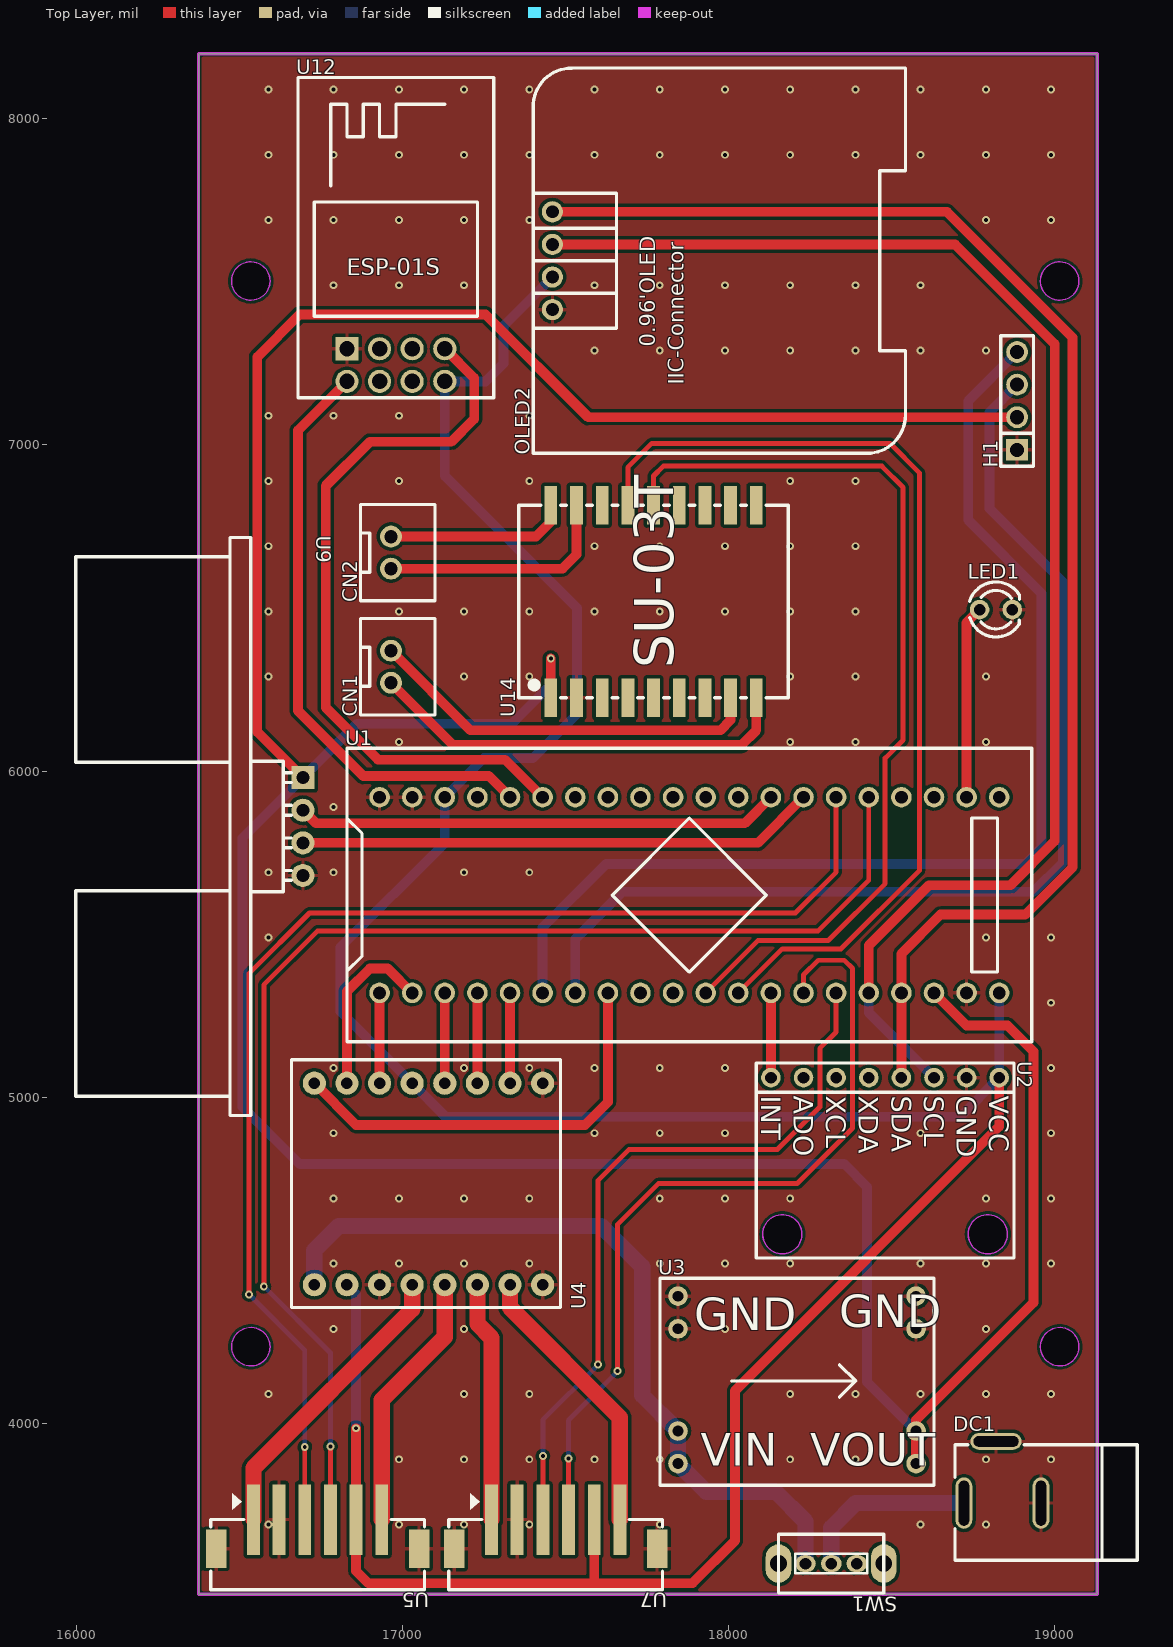
[diagram p0: Top Layer view]
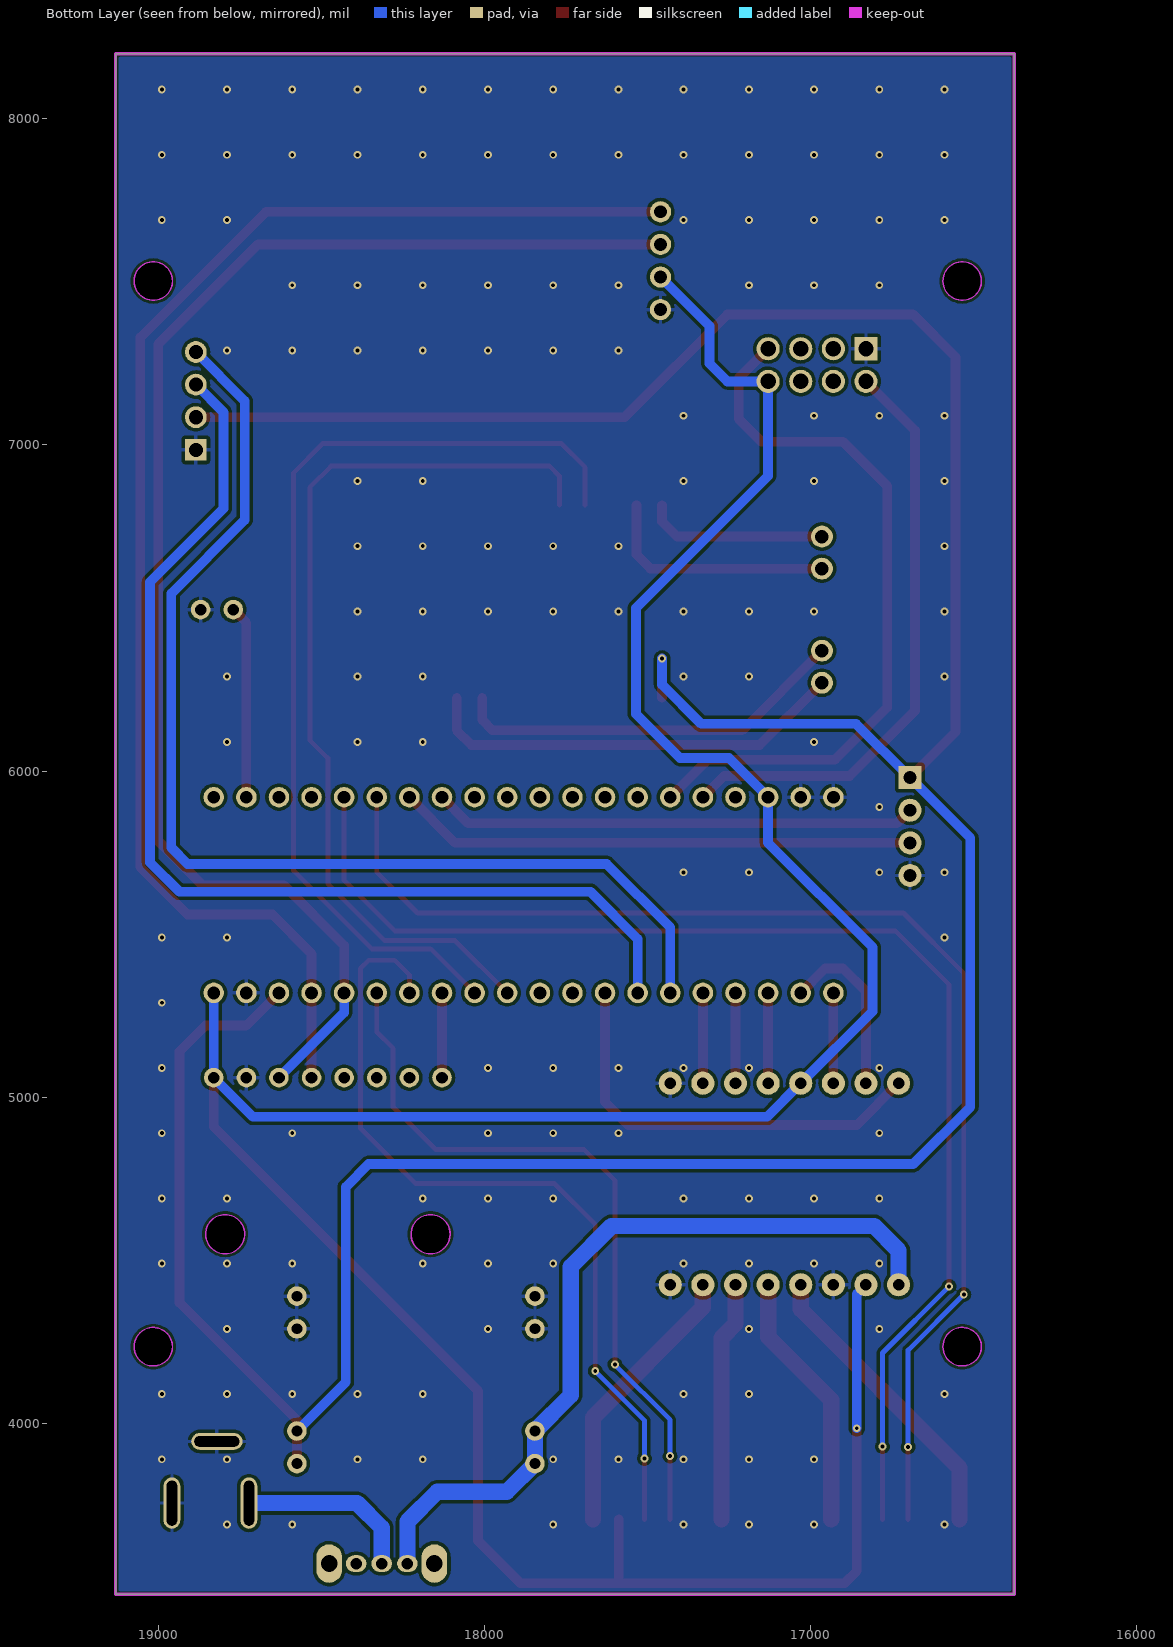
[diagram p1: Bottom Layer view, seen from below]
# Altium PCB MISC61229.pcbdoc
Units mil, origin at the board's own origin, x right, y up, seen from the top; angles counter-clockwise.
Board outline 2755.91 x 4724.41 mil, 2 copper layers (Top Layer, Bottom Layer), stack 62.206 mil thick; 16 components, 47 nets, 140 pads, 162 vias.

## Layer stack, top to bottom
Top Solder Mask Layer: solder mask 0.394, Dk 3.3
Top Layer: signal copper 1.379
Dielectric1: surface 59.449, FR4, Dk 4.5
Bottom Layer: signal copper 1.378
Bottom Solder Mask Layer: solder mask 0.394, Dk 3.3

## Board outline
16375,8200 16375,3475.59 19130.91,3475.59 19130.91,8200
cut-out: 16594.06,4235 cw(c16535,4235) 16475.94,4235 cw(c16535,4235)
cut-out: 16594.06,7502.72 cw(c16535,7502.72) 16475.94,7502.72 cw(c16535,7502.72)
cut-out: 19074.37,4235 cw(c19015.31,4235) 18956.26,4235 cw(c19015.31,4235)
cut-out: 19074.37,7502.72 cw(c19015.31,7502.72) 18956.26,7502.72 cw(c19015.31,7502.72)

## Design rules (kind name [scope] priority, off if disabled: settings)
BoardOutlineClearance copperThickness2oz_1 [All] p2 off: genericclearance=7.99 ignorepadtopadclearanceinfootprint=FALSE except(0: Arc-SplitContinuation Track-SplitContinuation SMDPad-SplitContinuation THPad-SplitContinuation Via-SplitContinuation Fill-SplitContinuation Region-SplitContinuation Poly-SplitContinuation Text-SplitContinuation Hole-SplitContinuation; 5.98: Arc-CutoutEdge Track-CutoutEdge SMDPad-CutoutEdge THPad-CutoutEdge Via-CutoutEdge Text-CutoutEdge; 6.9: Hole-OutlineEdge Hole-CutoutEdge; 10: Poly-OutlineEdge Poly-CutoutEdge; 11.81: Arc-OutlineEdge Track-OutlineEdge SMDPad-OutlineEdge THPad-OutlineEdge Via-OutlineEdge Fill-OutlineEdge Region-OutlineEdge Text-OutlineEdge Fill-CutoutEdge Region-CutoutEdge)
BoardOutlineClearance Plane_innerPlane_1 [All] p4 off: genericclearance=4.02 ignorepadtopadclearanceinfootprint=FALSE except(0: Arc-SplitContinuation Track-SplitContinuation SMDPad-SplitContinuation THPad-SplitContinuation Via-SplitContinuation Fill-SplitContinuation Region-SplitContinuation Poly-SplitContinuation Text-SplitContinuation Hole-SplitContinuation; 5.98: Arc-CutoutEdge Track-CutoutEdge SMDPad-CutoutEdge THPad-CutoutEdge Via-CutoutEdge Text-CutoutEdge; 6.9: Hole-OutlineEdge Hole-CutoutEdge; 10: Poly-OutlineEdge Poly-CutoutEdge; 11.81: Arc-OutlineEdge Track-OutlineEdge SMDPad-OutlineEdge THPad-OutlineEdge Via-OutlineEdge Fill-OutlineEdge Region-OutlineEdge Text-OutlineEdge Fill-CutoutEdge Region-CutoutEdge)
BoardOutlineClearance Copper_copperRegion_1 [All] p6 off: genericclearance=4.02 ignorepadtopadclearanceinfootprint=FALSE except(0: Arc-SplitContinuation Track-SplitContinuation SMDPad-SplitContinuation THPad-SplitContinuation Via-SplitContinuation Fill-SplitContinuation Region-SplitContinuation Poly-SplitContinuation Text-SplitContinuation Hole-SplitContinuation; 5.98: Arc-CutoutEdge Track-CutoutEdge SMDPad-CutoutEdge THPad-CutoutEdge Via-CutoutEdge Text-CutoutEdge; 6.9: Hole-OutlineEdge Hole-CutoutEdge; 10: Poly-OutlineEdge Poly-CutoutEdge; 11.81: Arc-OutlineEdge Track-OutlineEdge SMDPad-OutlineEdge THPad-OutlineEdge Via-OutlineEdge Fill-OutlineEdge Region-OutlineEdge Text-OutlineEdge Fill-CutoutEdge Region-CutoutEdge)
BoardOutlineClearance Copper_copperRegion_copperThickness1oz_1 [All] p8 off: genericclearance=4.02 ignorepadtopadclearanceinfootprint=FALSE except(0: Arc-SplitContinuation Track-SplitContinuation SMDPad-SplitContinuation THPad-SplitContinuation Via-SplitContinuation Fill-SplitContinuation Region-SplitContinuation Poly-SplitContinuation Text-SplitContinuation Hole-SplitContinuation; 5.98: Arc-CutoutEdge Track-CutoutEdge SMDPad-CutoutEdge THPad-CutoutEdge Via-CutoutEdge Text-CutoutEdge; 6.9: Hole-OutlineEdge Hole-CutoutEdge; 10: Poly-OutlineEdge Poly-CutoutEdge; 11.81: Arc-OutlineEdge Track-OutlineEdge SMDPad-OutlineEdge THPad-OutlineEdge Via-OutlineEdge Fill-OutlineEdge Region-OutlineEdge Text-OutlineEdge Fill-CutoutEdge Region-CutoutEdge)
BoardOutlineClearance Copper_copperRegion_Copper_copperRegion_1 [All] p10 off: genericclearance=4.02 ignorepadtopadclearanceinfootprint=FALSE except(0: Arc-SplitContinuation Track-SplitContinuation SMDPad-SplitContinuation THPad-SplitContinuation Via-SplitContinuation Fill-SplitContinuation Region-SplitContinuation Poly-SplitContinuation Text-SplitContinuation Hole-SplitContinuation; 5.98: Arc-CutoutEdge Track-CutoutEdge SMDPad-CutoutEdge THPad-CutoutEdge Via-CutoutEdge Text-CutoutEdge; 6.9: Hole-OutlineEdge Hole-CutoutEdge; 10: Poly-OutlineEdge Poly-CutoutEdge; 11.81: Arc-OutlineEdge Track-OutlineEdge SMDPad-OutlineEdge THPad-OutlineEdge Via-OutlineEdge Fill-OutlineEdge Region-OutlineEdge Text-OutlineEdge Fill-CutoutEdge Region-CutoutEdge)
BoardOutlineClearance copperThickness1oz_1 [All] p12: genericclearance=4.02 ignorepadtopadclearanceinfootprint=FALSE except(0: Arc-SplitContinuation Track-SplitContinuation SMDPad-SplitContinuation THPad-SplitContinuation Via-SplitContinuation Fill-SplitContinuation Region-SplitContinuation Poly-SplitContinuation Text-SplitContinuation Hole-SplitContinuation; 5.98: Arc-CutoutEdge Track-CutoutEdge SMDPad-CutoutEdge THPad-CutoutEdge Via-CutoutEdge Text-CutoutEdge; 6.9: Hole-OutlineEdge Hole-CutoutEdge; 10: Poly-OutlineEdge Poly-CutoutEdge; 11.81: Arc-OutlineEdge Track-OutlineEdge SMDPad-OutlineEdge THPad-OutlineEdge Via-OutlineEdge Fill-OutlineEdge Region-OutlineEdge Text-OutlineEdge Fill-CutoutEdge Region-CutoutEdge)
Clearance copperThickness2oz [All] p1 off: gap=7.99 ignorepadtopadclearanceinfootprint=FALSE except(5.98: SMDPad-Track SMDPad-SMDPad THPad-Track SMDPad-THPad THPad-THPad Track-Via SMDPad-Via THPad-Via Via-Via Fill-SMDPad Region-SMDPad Fill-THPad Region-THPad Fill-Via Region-Via Fill-Fill Fill-Region Region-Region Arc-Track Arc-SMDPad Arc-THPad Arc-Via Fill-Arc Region-Arc Arc-Arc Text-Track SMDPad-Text Text-THPad Text-Via Fill-Text Region-Text Arc-Text Text-Text; 6.9: Hole-Track Hole-SMDPad Hole-THPad Hole-Via Fill-Hole Region-Hole Hole-Arc Hole-Text; 10: Poly-Track Poly-SMDPad Poly-THPad Poly-Via Poly-Fill Poly-Region Poly-Poly Poly-Arc Poly-Text Poly-Hole; 11.81: Fill-Track Region-Track)
Clearance Plane_innerPlane [All] p3 off: gap=4.02 ignorepadtopadclearanceinfootprint=FALSE except(5.98: SMDPad-Track SMDPad-SMDPad THPad-Track SMDPad-THPad THPad-THPad Track-Via SMDPad-Via THPad-Via Via-Via Fill-SMDPad Region-SMDPad Fill-THPad Region-THPad Fill-Via Region-Via Fill-Fill Fill-Region Region-Region Arc-Track Arc-SMDPad Arc-THPad Arc-Via Fill-Arc Region-Arc Arc-Arc Text-Track SMDPad-Text Text-THPad Text-Via Fill-Text Region-Text Arc-Text Text-Text; 6.9: Hole-Track Hole-SMDPad Hole-THPad Hole-Via Fill-Hole Region-Hole Hole-Arc Hole-Text; 10: Poly-Track Poly-SMDPad Poly-THPad Poly-Via Poly-Fill Poly-Region Poly-Poly Poly-Arc Poly-Text Poly-Hole; 11.81: Fill-Track Region-Track)
Clearance Copper_copperRegion [All] p5 off: gap=4.02 ignorepadtopadclearanceinfootprint=FALSE except(5.98: SMDPad-Track SMDPad-SMDPad THPad-Track SMDPad-THPad THPad-THPad Track-Via SMDPad-Via THPad-Via Via-Via Fill-SMDPad Region-SMDPad Fill-THPad Region-THPad Fill-Via Region-Via Fill-Fill Fill-Region Region-Region Arc-Track Arc-SMDPad Arc-THPad Arc-Via Fill-Arc Region-Arc Arc-Arc Text-Track SMDPad-Text Text-THPad Text-Via Fill-Text Region-Text Arc-Text Text-Text; 6.9: Hole-Track Hole-SMDPad Hole-THPad Hole-Via Fill-Hole Region-Hole Hole-Arc Hole-Text; 10: Poly-Track Poly-SMDPad Poly-THPad Poly-Via Poly-Fill Poly-Region Poly-Poly Poly-Arc Poly-Text Poly-Hole; 11.81: Fill-Track Region-Track)
Clearance Copper_copperRegion_copperThickness1oz [All] p7 off: gap=4.02 ignorepadtopadclearanceinfootprint=FALSE except(5.98: SMDPad-Track SMDPad-SMDPad THPad-Track SMDPad-THPad THPad-THPad Track-Via SMDPad-Via THPad-Via Via-Via Fill-SMDPad Region-SMDPad Fill-THPad Region-THPad Fill-Via Region-Via Fill-Fill Fill-Region Region-Region Arc-Track Arc-SMDPad Arc-THPad Arc-Via Fill-Arc Region-Arc Arc-Arc Text-Track SMDPad-Text Text-THPad Text-Via Fill-Text Region-Text Arc-Text Text-Text; 6.9: Hole-Track Hole-SMDPad Hole-THPad Hole-Via Fill-Hole Region-Hole Hole-Arc Hole-Text; 10: Poly-Track Poly-SMDPad Poly-THPad Poly-Via Poly-Fill Poly-Region Poly-Poly Poly-Arc Poly-Text Poly-Hole; 11.81: Fill-Track Region-Track)
Clearance Copper_copperRegion_Copper_copperRegion [All] p9 off: gap=4.02 ignorepadtopadclearanceinfootprint=FALSE except(5.98: SMDPad-Track SMDPad-SMDPad THPad-Track SMDPad-THPad THPad-THPad Track-Via SMDPad-Via THPad-Via Via-Via Fill-SMDPad Region-SMDPad Fill-THPad Region-THPad Fill-Via Region-Via Fill-Fill Fill-Region Region-Region Arc-Track Arc-SMDPad Arc-THPad Arc-Via Fill-Arc Region-Arc Arc-Arc Text-Track SMDPad-Text Text-THPad Text-Via Fill-Text Region-Text Arc-Text Text-Text; 6.9: Hole-Track Hole-SMDPad Hole-THPad Hole-Via Fill-Hole Region-Hole Hole-Arc Hole-Text; 10: Poly-Track Poly-SMDPad Poly-THPad Poly-Via Poly-Fill Poly-Region Poly-Poly Poly-Arc Poly-Text Poly-Hole; 11.81: Fill-Track Region-Track)
Clearance copperThickness1oz [All] p11: gap=4.02 ignorepadtopadclearanceinfootprint=FALSE except(5.98: SMDPad-Track SMDPad-SMDPad THPad-Track SMDPad-THPad THPad-THPad Track-Via SMDPad-Via THPad-Via Via-Via Fill-SMDPad Region-SMDPad Fill-THPad Region-THPad Fill-Via Region-Via Fill-Fill Fill-Region Region-Region Arc-Track Arc-SMDPad Arc-THPad Arc-Via Fill-Arc Region-Arc Arc-Arc Text-Track SMDPad-Text Text-THPad Text-Via Fill-Text Region-Text Arc-Text Text-Text; 6.9: Hole-Track Hole-SMDPad Hole-THPad Hole-Via Fill-Hole Region-Hole Hole-Arc Hole-Text; 10: Poly-Track Poly-SMDPad Poly-THPad Poly-Via Poly-Fill Poly-Region Poly-Poly Poly-Arc Poly-Text Poly-Hole; 11.81: Fill-Track Region-Track)
DiffPairsRouting differentialPair [All] p1: maxlimit=6 minlimit=6 mostfreqgap=6 toplayer_minwidth=5 toplayer_prefwidth=10 toplayer_maxwidth=100 toplayer_mingap=6 toplayer_prefgap=6 toplayer_maxgap=6 bottomlayer_minwidth=5 bottomlayer_prefwidth=10 bottomlayer_maxwidth=100 bottomlayer_mingap=6 bottomlayer_prefgap=6 bottomlayer_maxgap=6 maxuncoupledlength=10
HoleToHoleClearance otherClearance [All] p1: gap=11.81 allowstackedmicrovias=TRUE
Length netLength [All] p1: minlimit=0 maxlimit=0
PasteMaskExpansion pasteMaskExpansion [All] p1: expansion=0
PlaneConnect innerPlane [All] p1: planeconnectstyle=Relief reliefexpansion=20 reliefentries=4 reliefconductorwidth=10 reliefairgap=10
PolygonConnect copperRegion_copperThickness1oz [All] p1 off: connectstyle=Relief reliefconductorwidth=10 reliefentries=4 polygonreliefangle="90 Angle" airgapwidth=10 via.connectstyle=Relief via.reliefconductorwidth=10 via.reliefentries=4 via.polygonreliefangle="90 Angle" via.airgapwidth=10
PolygonConnect copperRegion_Copper_copperRegion [All] p2 off: connectstyle=Relief reliefconductorwidth=10 reliefentries=4 polygonreliefangle="90 Angle" airgapwidth=10 via.connectstyle=Relief via.reliefconductorwidth=10 via.reliefentries=4 via.polygonreliefangle="90 Angle" via.airgapwidth=10
PolygonConnect copperRegion [All] p3: connectstyle=Relief reliefconductorwidth=10 reliefentries=4 polygonreliefangle="90 Angle" airgapwidth=10 via.connectstyle=Relief via.reliefconductorwidth=10 via.reliefentries=4 via.polygonreliefangle="90 Angle" via.airgapwidth=10
RoutingVias viaSize [All] p1: holewidth=12.01 width=24.02 viastyle="Through Hole" minholewidth=11.81 minwidth=19.68 maxholewidth=248.03 maxwidth=393.7
SolderMaskExpansion solderMaskExpansion [IsVia] p1: expansion=-1000 istentingtop=TRUE
SolderMaskExpansion solderMaskExpansion [All] p2: expansion=2 istentingtop=FALSE
Width copperThickness2oz_2 [All] p1 off: maxlimit=100 minlimit=8 preferedwidth=10
Width copperThickness1oz_2 [All] p2: maxlimit=100 minlimit=5 preferedwidth=10

## Components (designator, comment, footprint, x,y, rotation, side; value= is the part's Value field where it differs from the comment)
CN1 "XH2.54*2P_through-hole" CONN-TH_2P-P2.50-XH2.54-2P 16965,6320 r90 top
CN2 "XH2.54*2P_through-hole" CONN-TH_2P-P2.50-XH2.54-2P 16965,6670 r90 top
DC1 "" DC-2.0 18845,3745 r0 top
H1 "" HDR-TH_4P-P2.54-V-M 18884.82,7135.12 r90 top
LED1 "" LED_TH-3mm 18820,6495 r0 top
OLED2 "" 0.96OLED_4P 17460,7565 r90 top
SW1 "" 拨动开关 18320,3570 r180 top
U1 "STM32F103C8T6-Card" CONN-TH_L53.3-W22.9_STM32F103C8T6-CARD 17880,5620 r0 top
U2 "MPU6050 module" MPU6050 18480,5060 r270 top
U3 "" MP1584主控 17845,4390 r0 top
U4 "" tb6612 16730,4425 r90 top
U5 "MXPH-2.0-06P-LT1-0-A" CONN-SMD_6P-P2.00_MXPH-2.0-6P-LT1-0-A 16740,3660 r180 top
U7 "MXPH-2.0-06P-LT1-0-A" CONN-SMD_6P-P2.00_MXPH-2.0-6P-LT1-0-A 17470,3660 r180 top
U9 "HC-SR04" TH_HC-SR04V 16695,5830 r270 top
U12 "ESP-01S" WIFIM-TH_ESP-01S 16980,7245 r0 top
U14 "" SU-03T 18085,6520 r90 top

## Footprints (in the part's own frame and the unit in brackets; to place one, negate y for a bottom-side part, rotate by r counter-clockwise, add the part's x,y. Pads: shape width x height; smd on the part's side, far side on the other; paste and mask are expansions set on the pad)
0.96OLED_4P [mm]
  round 1.65 hole 1 copper offset 0,0: 1(-3.81,-0.001) 2(-1.27,0.002) 3(1.27,0.002) 4(3.81,0.002)
  silkscreen extent -15,-27.5 15,1.5
CONN-SMD_6P-P2.00_MXPH-2.0-6P-LT1-0-A [mm]
  rect 1x5.5 smd paste+0 mask+0.05: 1(5,-1.14) 2(3,-1.14) 3(1,-1.14) 4(-1,-1.14) 5(-3,-1.14) 6(-5,-1.14)
  rect 1.6x3 smd paste+0 mask+0.05: 7(-7.9,1.14) 8(7.9,1.14)
  silkscreen extent -8.32,-3.17 8.32,4.32
CONN-TH_2P-P2.50-XH2.54-2P [mm]
  round 1.7 hole 1.05 paste+0 mask+0.05: 1(1.25,0) 2(-1.25,0)
  silkscreen extent -3.75,-3.42 3.75,2.37
CONN-TH_L53.3-W22.9_STM32F103C8T6-CARD [mm]
  round 1.6 hole 1: 1(-24.13,-7.62) 2(-21.59,-7.62) 3(-19.05,-7.62) 4(-16.51,-7.62) 5(-13.97,-7.62) 6(-11.43,-7.62) 7(-8.89,-7.62) 8(-6.35,-7.62) 9(-3.81,-7.62) 10(-1.27,-7.62) 11(1.27,-7.62) 12(3.81,-7.62) 13(6.35,-7.62) 14(8.89,-7.62) 15(11.43,-7.62) 16(13.97,-7.62) 17(16.51,-7.62) 18(19.05,-7.62) 19(21.59,-7.62) 20(24.13,-7.62) 21(24.13,7.62) 22(21.59,7.62) 23(19.05,7.62) 24(16.51,7.62) 25(13.97,7.62) 26(11.43,7.62) 27(8.89,7.62) 28(6.35,7.62) 29(3.81,7.62) 30(1.27,7.62) 31(-1.27,7.62) 32(-3.81,7.62) 33(-6.35,7.62) 34(-8.89,7.62) 35(-11.43,7.62) 36(-13.97,7.62) 37(-16.51,7.62) 38(-19.05,7.62) 39(-21.59,7.62) 40(-24.13,7.62)
  silkscreen extent -26.67,-11.43 26.67,11.43
DC-2.0 [mil]
  oval 157.5x51.2 hole 31.5 slot 137.8 at 0 deg paste+0 mask+2: 2(-24.7,199.5)
  oval 51.2x157.5 hole 31.5 slot 137.8 at 90 deg paste+0 mask+2: 3(113.1,10.5) 4(-123.1,10.5)
  silkscreen extent -151,-165 408,190
HDR-TH_4P-P2.54-V-M [mm]
  rect 1.7x1.7 hole 1.1: 1(-3.81,0)
  round 1.7 hole 1.1: 2(-1.27,0) 3(1.27,0) 4(3.81,0)
  silkscreen extent -5.08,-1.27 5.08,1.27
LED_TH-3mm [mil]
  round 60 hole 36 paste+0 mask+2: 1(-50,0) 2(50,0)
  silkscreen extent -81,-84 72,85
MP1584主控 [mil]
  round 60 hole 33: 1(0,-100) 1(0,0) 2(0,-513.4) 2(0,-413.39) 3(730,-513.4) 3(730,-413.39) 4(730,-100) 4(730,0)
  silkscreen extent -55,-580 785,55
MPU6050 [mil]
  round 60 hole 36: 1(0,350) 2(0,250) 3(0,150) 4(0,50) 5(0,-50) 6(0,-150) 7(0,-250) 8(0,-350)
  Board Outline Layer circle w0.1: c480,315 r60
  Board Outline Layer circle w0.1: c480,-315 r60
  Board Outline Layer region: 480,375 506.03,369.06 526.91,352.41 538.5,328.35 538.5,301.65 526.91,277.59 506.03,260.94 480,255 480,255 453.97,260.94 433.09,277.59 421.5,301.65 421.5,328.35 433.09,352.41 453.97,369.06 480,375
  Board Outline Layer region: 480,375 486.72,374.62 493.35,373.5 499.82,371.63 506.03,369.06 511.92,365.8 517.41,361.91 522.43,357.43 526.91,352.41 530.8,346.92 534.06,341.03 536.63,334.82 538.5,328.35 539.62,321.72 540,315 539.62,308.28 538.5,301.65 536.63,295.18 534.06,288.97 530.8,283.08 526.91,277.59 522.43,272.57 517.41,268.09 511.92,264.2 506.03,260.94 499.82,258.37 493.35,256.5 486.72,255.38 480,255 473.28,255.38 466.65,256.5 460.18,258.37 453.97,260.94 448.08,264.2 442.59,268.09 437.57,272.57 433.09,277.59 429.2,283.08 425.94,288.97 423.37,295.18 421.5,301.65 420.38,308.28 420,315 420.38,321.72 421.5,328.35 423.37,334.82 425.94,341.03 429.2,346.92 433.09,352.41 437.57,357.43 442.59,361.91 448.08,365.8 453.97,369.06 460.18,371.63 466.65,373.5 473.28,374.62
  Board Outline Layer region: 480,-255 506.03,-260.94 526.91,-277.59 538.5,-301.65 538.5,-328.35 526.91,-352.41 506.03,-369.06 480,-375 480,-375 453.97,-369.06 433.09,-352.41 421.5,-328.35 421.5,-301.65 433.09,-277.59 453.97,-260.94 480,-255
  Board Outline Layer region: 480,-255 486.72,-255.38 493.35,-256.5 499.82,-258.37 506.03,-260.94 511.92,-264.2 517.41,-268.09 522.43,-272.57 526.91,-277.59 530.8,-283.08 534.06,-288.97 536.63,-295.18 538.5,-301.65 539.62,-308.28 540,-315 539.62,-321.72 538.5,-328.35 536.63,-334.82 534.06,-341.03 530.8,-346.92 526.91,-352.41 522.43,-357.43 517.41,-361.91 511.92,-365.8 506.03,-369.06 499.82,-371.63 493.35,-373.5 486.72,-374.62 480,-375 473.28,-374.62 466.65,-373.5 460.18,-371.63 453.97,-369.06 448.08,-365.8 442.59,-361.91 437.57,-357.43 433.09,-352.41 429.2,-346.92 425.94,-341.03 423.37,-334.82 421.5,-328.35 420.38,-321.72 420,-315 420.38,-308.28 421.5,-301.65 423.37,-295.18 425.94,-288.97 429.2,-283.08 433.09,-277.59 437.57,-272.57 442.59,-268.09 448.08,-264.2 453.97,-260.94 460.18,-258.37 466.65,-256.5 473.28,-255.38
  Multi-Layer board cut-out: 480,375 506.03,369.06 526.91,352.41 538.5,328.35 538.5,301.65 526.91,277.59 506.03,260.94 480,255 480,255 453.97,260.94 433.09,277.59 421.5,301.65 421.5,328.35 433.09,352.41 453.97,369.06 480,375
  Multi-Layer board cut-out: 480,-255 506.03,-260.94 526.91,-277.59 538.5,-301.65 538.5,-328.35 526.91,-352.41 506.03,-369.06 480,-375 480,-375 453.97,-369.06 433.09,-352.41 421.5,-328.35 421.5,-301.65 433.09,-277.59 453.97,-260.94 480,-255
  silkscreen extent -45,-395 553,395
SU-03T [mm]
  rect 3x1 smd: 1(-7.5,16) 2(-7.5,14) 3(-7.5,12) 4(-7.5,10) 5(-7.5,8) 6(-7.5,6) 7(-7.5,4) 8(-7.5,2) 9(-7.5,0) 10(7.5,0) 11(7.5,2) 12(7.5,4) 13(7.5,6) 14(7.5,8) 15(7.5,10) 16(7.5,12) 17(7.5,14) 18(7.5,16)
  silkscreen extent -7.5,-2.5 7.5,18.5
tb6612 [mm]
  round 1.8 hole 0.9: 1(0,0) 2(0,-2.54) 3(0,-5.08) 4(0,-7.62) 5(0,-10.16) 6(0,-12.7) 7(0,-15.24) 8(0,-17.78) 9(15.697,-17.78) 10(15.697,-15.24) 11(15.697,-12.7) 12(15.697,-10.16) 13(15.697,-7.62) 14(15.697,-5.08) 15(15.697,-2.54) 16(15.697,0)
  silkscreen extent -1.78,-19.18 17.53,1.78
TH_HC-SR04V [mm]
  rect 1.8x1.8 hole 1.001: 1(-3.81,0)
  round 1.8 hole 1.001: 2(-1.27,0) 3(1.27,0) 4(3.81,0)
  silkscreen extent -22.5,-17.7 22.5,-0.89
WIFIM-TH_ESP-01S [mm]
  rect 1.8x1.8 hole 1.2: 1(-3.81,1.27)
  round 1.8 hole 1.2: 2(-1.27,1.27) 3(1.27,1.27) 4(3.81,1.27) 5(3.81,-1.27) 6(1.27,-1.27) 7(-1.27,-1.27) 8(-3.81,-1.27)
  silkscreen extent -7.62,-2.54 7.62,22.4
拨动开关 [mil]
  oval 63x51.2 hole 35.4 paste+0 mask+2: 1(-73.4,0) 2(5,0) 3(84,0)
  oval 78.7x118.1 hole 51.2 paste+0 mask+2: 4(166.7,0) 5(-156.1,0)
  silkscreen extent -156,-90 167,90

## Via types
v1: diameter 24.02, hole 12, Top Layer to Bottom Layer, 162 vias

## Nets (pads, with @x,y where several pads share a name; then routed paths per layer and width w, separated by ;. In a path a pad name is that pad's centre, name@x,y a point inside that pad or via, vN(x,y) a via of type N, cw(c..) or ccw(c..) an arc to the next point about the centre after c; other vN are vias at no path point)
$1N17402: DC1.4 SW1.2 | length 548.2
  Bottom Layer w50: SW1.2 18315,3680 18390.5,3755.5 DC1.4
$1N17403: CN1.1 U14.8 | length 1223.8
  Top Layer w30: CN1.1 17209.22,6125 17975,6125 18006.26,6156.26 U14.8
$1N17404: CN1.2 U14.9 | length 1317.4
  Top Layer w30: CN1.2 17155.78,6080 18040,6080 18085,6125 U14.9
$1N17405: CN2.1 U14.18 | length 559.3
  Top Layer w30: CN2.1 17409.22,6719.22 17455.08,6765.08 U14.18
$1N17406: CN2.2 U14.17 | length 738.1
  Top Layer w30: CN2.2 17490.78,6620.78 17533.82,6663.82 U14.17
+5V: H1.2 U1.18 U3.3 U9.1 U14.1 | length 10646.1
  Top Layer w30: U9.1 16555,6120 16555,7270 16685,7400 17255,7400 17569.88,7085.12 H1.2 ; v1(17455,6345) 17455,6224.8 U14.1 ; U3.3@18575,3876.6 18575,3976.61 18575,4010 18935,4370 18935,5140 18855,5220 18730,5220 U1.18
  Bottom Layer w30: v1(17455,6345) 17455,6265 17335,6145 16860,6145 U9.1 16510,5795 16510,4970 16685,4795 18355,4795 18425,4725 18425,4126.61 U3.3@18575,3976.61
AO1: U4.4 U5.1 | length 921.8
  Top Layer w50: U5.1 16543.15,3863.15 17030,4350 U4.4
AO2: U4.5 U5.6 | length 800.1
  Top Layer w50: U5.6 16936.85,4071.85 17130,4265 U4.5
BO1: U4.7 U7.6 | length 859.6
  Top Layer w50: U4.7 17330,4355 17666.85,4018.15 U7.6
BO2: U4.6 U7.1 | length 738
  Top Layer w50: U4.6 17230,4305 17273.15,4261.85 U7.1
GND: DC1.2 DC1.3 H1.1 LED1.2 OLED2.1 U1.19 U1.39 U1.40 U2.2 U3.1 U3.4 U4.3 U4.8 U4.9 U5.2 U5.7 U5.8 U7.2 U7.7 U7.8 U9.4 U12.1 U14.2
  other v1: 16589.1,3689.69 16989.1,3689.69 17189.1,3689.69 17389.1,3689.69 17789.1,3689.69 18589.1,3689.69 18789.1,3689.69 16989.1,3889.69 17189.1,3889.69 17389.1,3889.69 17589.1,3889.69 17789.1,3889.69 18189.1,3889.69 18389.1,3889.69 18789.1,3889.69 18989.1,3889.69 16589.1,4089.69 17189.1,4089.69 17389.1,4089.69 18189.1,4089.69 18389.1,4089.69 18589.1,4089.69 18789.1,4089.69 18989.1,4089.69 16789.1,4289.69 17189.1,4289.69 17989.1,4289.69 18789.1,4289.69 16789.1,4489.69 16989.1,4489.69 17189.1,4489.69 17389.1,4489.69 17789.1,4489.69 17989.1,4489.69 18189.1,4489.69 18589.1,4489.69 18789.1,4489.69 18989.1,4489.69 16789.1,4689.69 16989.1,4689.69 17189.1,4689.69 17389.1,4689.69 17789.1,4689.69 17989.1,4689.69 18189.1,4689.69 18789.1,4689.69 18989.1,4689.69 16789.1,4889.69 17589.1,4889.69 17789.1,4889.69 17989.1,4889.69 18589.1,4889.69 18989.1,4889.69 16789.1,5089.69 17189.1,5089.69 17389.1,5089.69 17589.1,5089.69 17789.1,5089.69 17989.1,5089.69 18989.1,5089.69 18989.1,5289.69 16589.1,5489.69 18789.1,5489.69 18989.1,5489.69 16589.1,5689.69 16789.1,5689.69 17189.1,5689.69 17389.1,5689.69 16789.1,5889.69 16989.1,6089.69 18189.1,6089.69 18389.1,6089.69 18789.1,6089.69 16589.1,6289.69 17189.1,6289.69 17389.1,6289.69 18189.1,6289.69 18389.1,6289.69 18789.1,6289.69 16589.1,6489.69 16989.1,6489.69 17189.1,6489.69 17389.1,6489.69 17589.1,6489.69 17789.1,6489.69 17989.1,6489.69 18189.1,6489.69 18389.1,6489.69 16589.1,6689.69 17589.1,6689.69 17789.1,6689.69 17989.1,6689.69 18189.1,6689.69 18389.1,6689.69 16589.1,6889.69 16989.1,6889.69 17389.1,6889.69 18189.1,6889.69 18389.1,6889.69 16589.1,7089.69 16789.1,7089.69 16989.1,7089.69 17389.1,7089.69 17589.1,7289.69 17789.1,7289.69 17989.1,7289.69 18189.1,7289.69 18389.1,7289.69 18589.1,7289.69 18789.1,7289.69 16789.1,7489.69 16989.1,7489.69 17189.1,7489.69 17589.1,7489.69 17789.1,7489.69 17989.1,7489.69 18189.1,7489.69 18389.1,7489.69 18589.1,7489.69 16589.1,7689.69 16789.1,7689.69 16989.1,7689.69 17189.1,7689.69 17389.1,7689.69 18789.1,7689.69 18989.1,7689.69 16589.1,7889.69 16789.1,7889.69 16989.1,7889.69 17189.1,7889.69 17389.1,7889.69 17589.1,7889.69 17789.1,7889.69 17989.1,7889.69 18189.1,7889.69 18389.1,7889.69 18589.1,7889.69 18789.1,7889.69 18989.1,7889.69 16589.1,8089.69 16789.1,8089.69 16989.1,8089.69 17189.1,8089.69 17389.1,8089.69 17589.1,8089.69 17789.1,8089.69 17989.1,8089.69 18189.1,8089.69 18389.1,8089.69 18589.1,8089.69 18789.1,8089.69 18989.1,8089.69
NRST: U1.37
PA0: U1.25 U5.4 | length 3967.3
  Top Layer w15: v1(16575,4420) 16575,5345 16740,5510 18275,5510 18430,5665 U1.25 ; U5.4 v1(16779.37,3928.75)
  Bottom Layer w15: v1(16575,4420) 16779.37,4215.63 v1(16779.37,3928.75)
PA1: U1.26 U5.3 | length 3904.2
  Top Layer w15: v1(16530,4395) 16530,5380 16715,5565 18205,5565 18330,5690 U1.26 ; U5.3 v1(16700.63,3927.28)
  Bottom Layer w15: v1(16530,4395) 16700.63,4224.37 v1(16700.63,3927.28)
PA2: U1.27 U9.3 | length 1593
  Top Layer w30: U9.3 18090,5780 U1.27
PA3: U1.28 U9.2 | length 1484.7
  Top Layer w30: U9.2 16735,5840 18050,5840 U1.28
PA4: U1.29
PA5: U1.30
PA6: U1.31
PA7: U1.32
PA8: U1.5 U4.10 | length 277
  Top Layer w30: U4.10 U1.5
PA9: H1.4 U1.6 | length 3506.9
  Bottom Layer w30: U1.6 17430,5520 17625,5715 18910,5715 18960,5765 18960,6545 18735,6770 18735,7135.3 H1.4
PA10: H1.3 U1.7 | length 3350.8
  Bottom Layer w30: U1.7 17530,5485 17675,5630 18935,5630 19025,5720 19025,6580 18800,6805 18800,7100.3 H1.3
PA11: U1.8 U4.16 | length 1317
  Top Layer w30: U4.16 16858,4915 17560,4915 17630,4985 U1.8
PA12: U1.9
PA15: U1.10
PB0: U1.33
PB1: U1.34
PB3: U1.11 U14.14 | length 2820.6
  Top Layer w15: U14.14 17770.04,6905.04 17800,6935 18470,6935 18535,6870 18535,6095 18480,6040 18480,5655 18305,5480 18090,5480 U1.11
PB4: U1.12 U14.15 | length 3007.9
  Top Layer w15: U14.15 17691.3,6931.3 17765,7005 18495,7005 18585,6915 18585,5695 18345,5455 18165,5455 U1.12
PB5: U1.13 U2.8 | length 260
  Top Layer w30: U2.8 U1.13
PB6: U1.14 U7.4 | length 2533.7
  Top Layer w15: U7.4 v1(17509.37,3892.4) ; v1(17660,4160) 17660,4610 17785,4735 18210,4735 18380,4905 18380,5395 18355,5420 18275,5420 18230,5375 U1.14
  Bottom Layer w15: v1(17509.37,3892.4) 17509.37,4009.37 v1(17660,4160)
PB7: U1.15 U7.3 | length 2254.2
  Top Layer w15: U7.3 v1(17430.63,3899.46) ; v1(17600,4180) 17600,4745 17695,4840 18150,4840 18280,4970 18280,5150 18330,5200 U1.15
  Bottom Layer w15: v1(17430.63,3899.46) 17430.63,4010.63 v1(17600,4180)
PB8: OLED2.3 U1.16 U2.3 | length 4381.8
  Top Layer w30: OLED2.3@17459.95,7615 18695,7615 19000,7310 19000,5785 18865,5650 18615,5650 18430,5465 U1.16
  Bottom Layer w30: U1.16 18430,5260 U2.3
PB9: OLED2.4 U1.17 U2.4 | length 4394.3
  Top Layer w30: OLED2.4@17459.95,7715 18670,7715 19055,7330 19055,5705 18910,5560 18650,5560 18530,5440 U1.17 U2.4
PB10: U1.35 U12.4 | length 2251.1
  Top Layer w30: U12.4 17220,7205 17220,7080 17150,7010 16900,7010 16765,6875 16765,6195 16925,6035 17315,6035 U1.35
PB11: U1.36 U12.8 | length 1831.9
  Top Layer w30: U12.8 16680,7045 16680,6185 16880,5985 17265,5985 U1.36
PB12: U1.1 U4.14 | length 277
  Top Layer w30: U4.14 U1.1
PB13: U1.2 U4.15 | length 542.1
  Top Layer w30: U4.15 16830,5325 16900,5395 16955,5395 U1.2
PB14: U1.3 U4.12 | length 277
  Top Layer w30: U4.12 U1.3
PB15: U1.4 U4.11 | length 277
  Top Layer w30: U4.11 U1.4
PC13: LED1.1 U1.22 | length 591.6
  Top Layer w30: U1.22 18730,6455 LED1.1
PC14: U1.23
PC15: U1.24
VBAT: U1.21
VCC: OLED2.2 U1.20 U1.38 U2.1 U4.2 U4.13 U5.5 U7.5 U12.5 | length 9552.5
  Top Layer w30: v1(16858.11,3985) U5.5 16858.11,3546.89 16895,3510 17588.11,3510 ; U7.5 17588.11,3510 ; U2.1 18830,4910 18020,4100 18020,3640 17890,3510 17588.11,3510
  Bottom Layer w30: U4.2 16858.11,4396.89 v1(16858.11,3985) ; OLED2.2@17459.95,7515 17310,7365.05 17310,7250 17255,7195 U12.5 17130,6905 17535,6500 17535,6175 17400,6040 17250,6040 U1.38 17130,5780 16810,5460 16810,5263 U4.13 17133,4940 18710,4940 U2.1 U1.20
VM: SW1.3 U3.2 U4.1 | length 2435.4
  Bottom Layer w50: U4.1 16730,4530 16805,4605 17610,4605 17735,4480 17735,4086.61 17845,3976.61 17845,3876.6 17931.6,3790 18145,3790 18236,3699 SW1.3
pads on no net: SW1.1 SW1.4 SW1.5 U2.5 U2.6 U2.7 U12.2 U12.3 U12.6 U12.7 U14.3 U14.4 U14.5 U14.6 U14.7 U14.10 U14.11 U14.12 U14.13 U14.16

## Polygon pours and split planes (outlines as drawn)
GND on Bottom Layer (solid, remove dead copper, pour order 4): 3525,10310 3525,6145 7700,6145 7700,10310
GND on Top Layer (solid, remove dead copper, pour order 2): 3000,10480 3000,6065 7930,6065 7930,10480
GND on Top Layer (solid, remove dead copper, pour order 4): 14955,8895 14955,3000 20820,3000 20820,8895
GND on Bottom Layer (solid, remove dead copper, pour order 6): 15735,8510 15735,3020 19990,3020 19990,8510

## Keep-outs
Board Outline Layer:
  region: 16594.06,4235 cw(c16535,4235) 16475.94,4235 cw(c16535,4235)
  circle w0.1: c16535,4235 r59.06
  region: 16594.06,4235 16593.66,4228.14 16592.46,4221.38 16590.49,4214.8 16587.77,4208.5 16584.34,4202.55 16580.24,4197.04 16575.53,4192.04 16570.27,4187.63 16564.53,4183.86 16558.39,4180.77 16551.94,4178.43 16545.25,4176.84 16538.43,4176.04 16531.57,4176.04 16524.75,4176.84 16518.06,4178.43 16511.61,4180.77 16505.47,4183.86 16499.73,4187.63 16494.47,4192.04 16489.76,4197.04 16485.66,4202.55 16482.23,4208.5 16479.51,4214.8 16477.54,4221.38 16476.34,4228.14 16475.94,4235 16476.34,4241.86 16477.54,4248.62 16479.51,4255.2 16482.23,4261.5 16485.66,4267.45 16489.76,4272.96 16494.47,4277.96 16499.73,4282.37 16505.47,4286.14 16511.61,4289.23 16518.06,4291.57 16524.75,4293.16 16531.57,4293.96 16538.43,4293.96 16545.25,4293.16 16551.94,4291.57 16558.39,4289.23 16564.53,4286.14 16570.27,4282.37 16575.53,4277.96 16580.24,4272.96 16584.34,4267.45 16587.77,4261.5 16590.49,4255.2 16592.46,4248.62 16593.66,4241.86
  region: 16594.06,7502.72 cw(c16535,7502.72) 16475.94,7502.72 cw(c16535,7502.72)
  circle w0.1: c16535,7502.72 r59.06
  region: 16594.06,7502.72 16593.66,7495.86 16592.46,7489.1 16590.49,7482.52 16587.77,7476.21 16584.34,7470.27 16580.24,7464.76 16575.53,7459.76 16570.27,7455.35 16564.53,7451.57 16558.39,7448.49 16551.94,7446.14 16545.25,7444.56 16538.43,7443.76 16531.57,7443.76 16524.75,7444.56 16518.06,7446.14 16511.61,7448.49 16505.47,7451.57 16499.73,7455.35 16494.47,7459.76 16489.76,7464.76 16485.66,7470.27 16482.23,7476.21 16479.51,7482.52 16477.54,7489.1 16476.34,7495.86 16475.94,7502.72 16476.34,7509.57 16477.54,7516.34 16479.51,7522.91 16482.23,7529.22 16485.66,7535.17 16489.76,7540.68 16494.47,7545.67 16499.73,7550.09 16505.47,7553.86 16511.61,7556.94 16518.06,7559.29 16524.75,7560.87 16531.57,7561.67 16538.43,7561.67 16545.25,7560.87 16551.94,7559.29 16558.39,7556.94 16564.53,7553.86 16570.27,7550.09 16575.53,7545.67 16580.24,7540.68 16584.34,7535.17 16587.77,7529.22 16590.49,7522.91 16592.46,7516.34 16593.66,7509.57
  region: 19074.37,4235 cw(c19015.31,4235) 18956.26,4235 cw(c19015.31,4235)
  circle w0.1: c19015.31,4235 r59.06
  region: 19074.37,4235 19073.97,4228.14 19072.78,4221.38 19070.81,4214.8 19068.09,4208.5 19064.65,4202.55 19060.55,4197.04 19055.84,4192.04 19050.58,4187.63 19044.84,4183.86 19038.71,4180.77 19032.25,4178.43 19025.57,4176.84 19018.75,4176.04 19011.88,4176.04 19005.06,4176.84 18998.38,4178.43 18991.92,4180.77 18985.79,4183.86 18980.05,4187.63 18974.79,4192.04 18970.08,4197.04 18965.98,4202.55 18962.54,4208.5 18959.82,4214.8 18957.85,4221.38 18956.66,4228.14 18956.26,4235 18956.66,4241.86 18957.85,4248.62 18959.82,4255.2 18962.54,4261.5 18965.98,4267.45 18970.08,4272.96 18974.79,4277.96 18980.05,4282.37 18985.79,4286.14 18991.92,4289.23 18998.38,4291.57 19005.06,4293.16 19011.88,4293.96 19018.75,4293.96 19025.57,4293.16 19032.25,4291.57 19038.71,4289.23 19044.84,4286.14 19050.58,4282.37 19055.84,4277.96 19060.55,4272.96 19064.65,4267.45 19068.09,4261.5 19070.81,4255.2 19072.78,4248.62 19073.97,4241.86
  region: 19074.37,7502.72 cw(c19015.31,7502.72) 18956.26,7502.72 cw(c19015.31,7502.72)
  circle w0.1: c19015.31,7502.72 r59.06
  region: 19074.37,7502.72 19073.97,7495.86 19072.78,7489.1 19070.81,7482.52 19068.09,7476.21 19064.65,7470.27 19060.55,7464.76 19055.84,7459.76 19050.58,7455.35 19044.84,7451.57 19038.71,7448.49 19032.25,7446.14 19025.57,7444.56 19018.75,7443.76 19011.88,7443.76 19005.06,7444.56 18998.38,7446.14 18991.92,7448.49 18985.79,7451.57 18980.05,7455.35 18974.79,7459.76 18970.08,7464.76 18965.98,7470.27 18962.54,7476.21 18959.82,7482.52 18957.85,7489.1 18956.66,7495.86 18956.26,7502.72 18956.66,7509.57 18957.85,7516.34 18959.82,7522.91 18962.54,7529.22 18965.98,7535.17 18970.08,7540.68 18974.79,7545.67 18980.05,7550.09 18985.79,7553.86 18991.92,7556.94 18998.38,7559.29 19005.06,7560.87 19011.88,7561.67 19018.75,7561.67 19025.57,7560.87 19032.25,7559.29 19038.71,7556.94 19044.84,7553.86 19050.58,7550.09 19055.84,7545.67 19060.55,7540.68 19064.65,7535.17 19068.09,7529.22 19070.81,7522.91 19072.78,7516.34 19073.97,7509.57
  lines w10: 16375,3475.59 16375,8200 19130.91,8200 19130.91,3475.59 16375,3475.59

## Silkscreen, mask and mechanical layers (free items; w line width, h text height)
Mechanical Layer:
  circle w0.1: c16535,4235 r59.06
  circle w0.1: c16535,7502.72 r59.06
  circle w0.1: c19015.31,4235 r59.06
  circle w0.1: c19015.31,7502.72 r59.06